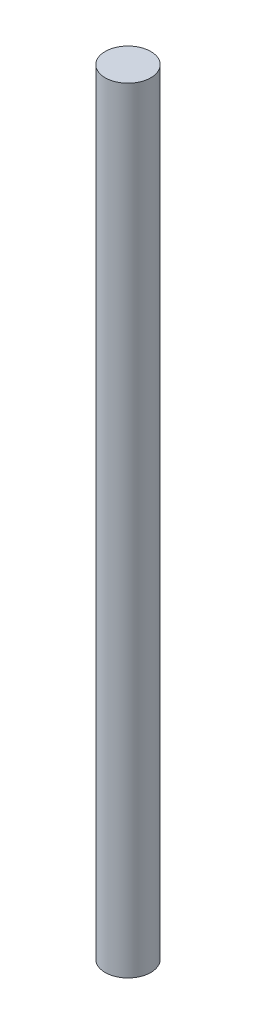
from build123d import *

# Parameters (mm, degrees)
SKETCH_1_R      = 1
EXTRUDE_1_DEPTH = 34


with BuildPart() as part:
    # 草图1 → 凸台-拉伸1 (new body)
    with BuildSketch(Plane(origin=(0, 0, 0), x_dir=(1, 0, 0), z_dir=(0, 1, 0))):
        with Locations(Location((0, 0, 0), (0, 0, 270))):
            Circle(SKETCH_1_R)
    extrude(amount=EXTRUDE_1_DEPTH)


solid = part.part
